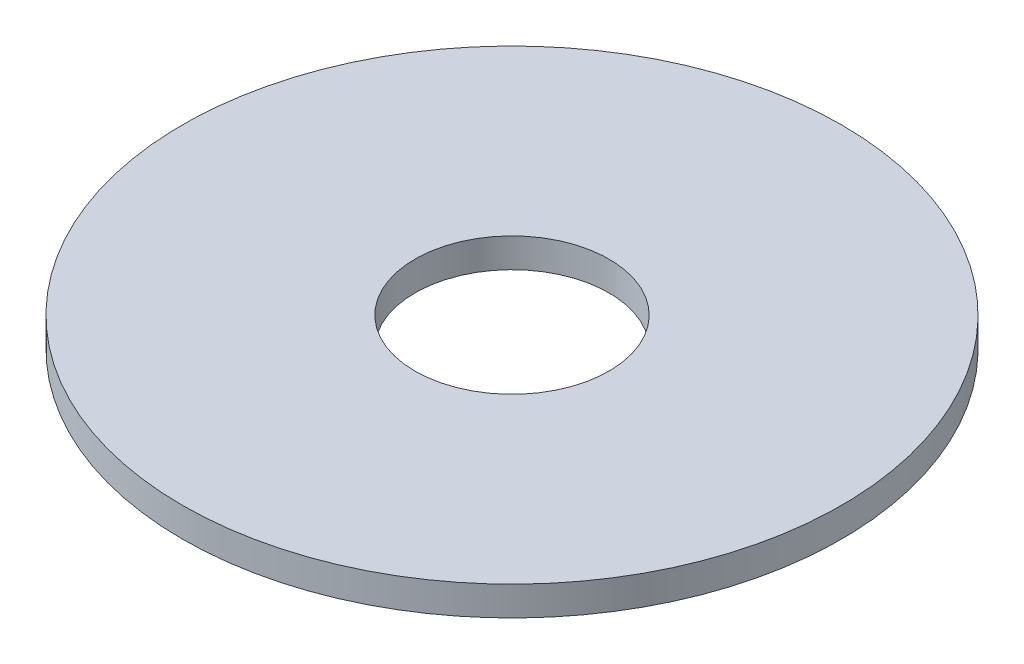
from build123d import *

# Parameters (mm, degrees)
SKETCH_1_R      = 45
SKETCH_1_R_2    = 13.25
EXTRUDE_1_DEPTH = 2


with BuildPart() as part:
    # 草图1 → 凸台-拉伸1 (new, symmetric)
    with BuildSketch(Plane(origin=(0, 0, 0), x_dir=(1, 0, 0), z_dir=(0, 1, 0))):
        with Locations(Location((0, 0, 0), (0, 0, 270))):
            Circle(SKETCH_1_R)
        with Locations(Location((0, 0, 0), (0, 0, 270))):
            Circle(SKETCH_1_R_2, mode=Mode.SUBTRACT)
    extrude(amount=EXTRUDE_1_DEPTH, both=True)


solid = part.part
